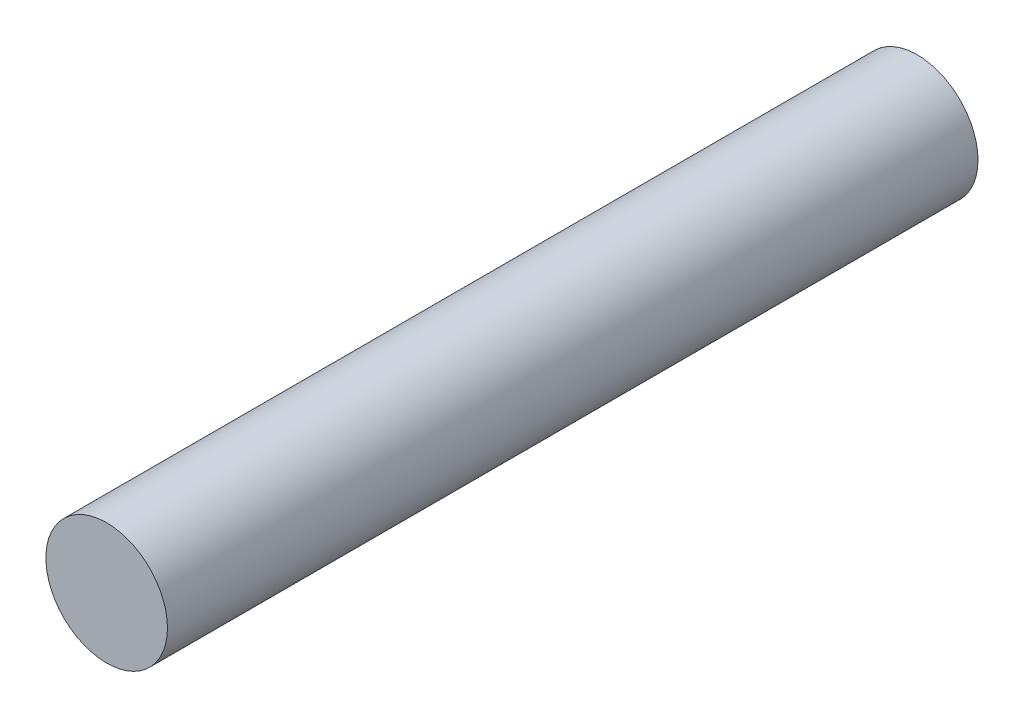
from build123d import *

# Parameters (mm, degrees)
SKETCH1_R    = 75
LENGTH_DEPTH = 1000


with BuildPart() as part:
    # Sketch1 → Length (new body)
    with BuildSketch(Plane.XY):
        Circle(SKETCH1_R)
    extrude(amount=LENGTH_DEPTH)


solid = part.part
